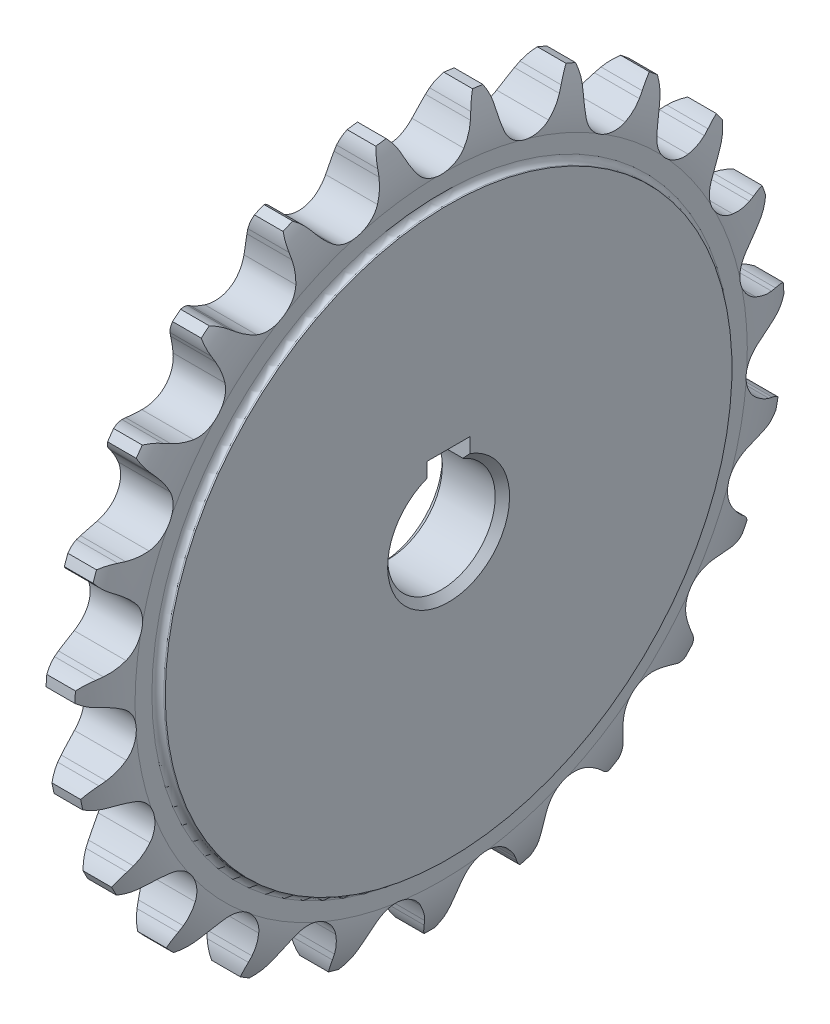
from build123d import *

# Parameters (mm, degrees)
CUT_EXTRUDE_1_DEPTH      = 4.685156443
PATTERN_CIRCULAR_1_COUNT = 23
SKETCH_4_W               = 6
SKETCH_4_H               = 3.126136458
CUT_EXTRUDE_2_DEPTH      = 71.578126957
CHAMFER_1_SIZE           = 1
CHAMFER_2_SIZE           = 1


with BuildPart() as part:
    # 草图1 → 旋转1 (revolve)
    with BuildSketch(Plane.XY, mode=Mode.PRIVATE) as revolve_1_sk:
        with BuildLine():
            Line((-4.685156443, 7.5), (-4.685156443, 39.5))
            Line((-4.685156443, 39.5), (-4.478175154, 39.5))
            ThreePointArc((-4.478175154, 39.5), (-3.892743663, 39.742493663), (-3.65025, 40.327925154))
            Line((-3.65025, 40.327925154), (-3.65025, 42.674032945))
            ThreePointArc((-3.65025, 42.674032945), (-3.305953661, 46.203405438), (-1.99925, 49.5))
            Line((-1.99925, 49.5), (1.99925, 49.5))
            ThreePointArc((1.99925, 49.5), (3.305953661, 46.203405438), (3.65025, 42.674032945))
            Line((3.65025, 42.674032945), (3.65025, 40.327925154))
            ThreePointArc((3.65025, 40.327925154), (3.892743663, 39.742493663), (4.478175154, 39.5))
            Line((4.478175154, 39.5), (4.685156443, 39.5))
            Line((4.685156443, 39.5), (4.685156443, 7.5))
            Line((4.685156443, 7.5), (-4.685156443, 7.5))
        make_face()
    revolve(revolve_1_sk.sketch.rotate(Axis((-6.35, 0, 0), (1, 0, 0)), 90), axis=Axis((-6.35, 0, 0), (1, 0, 0)))

    # 草图2 → 切除-拉伸1 (cut, symmetric)
    with BuildSketch(Plane(origin=(0, 0, 0), x_dir=(0, 0, -1), z_dir=(1, 0, 0))):
        with BuildLine():
            Line((4.588692581, 46.610285416), (4.899653292, 47.378261808))
            ThreePointArc((4.899653292, 47.378261808), (5.378614734, 48.306828579), (6.018529669, 49.132751812))
            ThreePointArc((6.018529669, 49.132751812), (0, 49.5), (-6.018529669, 49.132751812))
            ThreePointArc((-6.018529669, 49.132751812), (-5.378614734, 48.306828579), (-4.899653292, 47.378261808))
            Line((-4.899653292, 47.378261808), (-4.588692581, 46.610285416))
            ThreePointArc((-4.588692581, 46.610285416), (-3.973376288, 45.345046883), (-3.192395607, 44.174785433))
            ThreePointArc((-3.192395607, 44.174785433), (0, 42.604232945), (3.192395607, 44.174785433))
            ThreePointArc((3.192395607, 44.174785433), (3.973376288, 45.345046883), (4.588692581, 46.610285416))
        make_face()
    cut_extrude_1 = extrude(amount=CUT_EXTRUDE_1_DEPTH, both=True, mode=Mode.SUBTRACT)

    # 阵列(圆周)1: 切除-拉伸1 ×23 about axis
    pattern_circular_1_axis = Axis((0, 0, 0), (1, 0, 0))
    for i in range(1, PATTERN_CIRCULAR_1_COUNT):
        add(cut_extrude_1.rotate(pattern_circular_1_axis, i * 360 / PATTERN_CIRCULAR_1_COUNT), mode=Mode.SUBTRACT)

    # 草图4 → 切除-拉伸2 (cut, through all)
    with BuildSketch(Plane.ZY.offset(4.685156443)):
        with Locations((0, 8.436931771)):
            Rectangle(SKETCH_4_W, SKETCH_4_H)
    extrude(amount=-CUT_EXTRUDE_2_DEPTH, mode=Mode.SUBTRACT)

    # 倒角1
    chamfer_1_edges = [part.edges().sort_by_distance(p)[0] for p in [
        (-4.685156443, -7.5, 0),
    ]]
    chamfer(chamfer_1_edges, length=CHAMFER_1_SIZE)

    # 倒角2
    chamfer_2_edges = [part.edges().sort_by_distance(p)[0] for p in [
        (4.685156443, -7.5, 0),
    ]]
    chamfer(chamfer_2_edges, length=CHAMFER_2_SIZE)


solid = part.part
